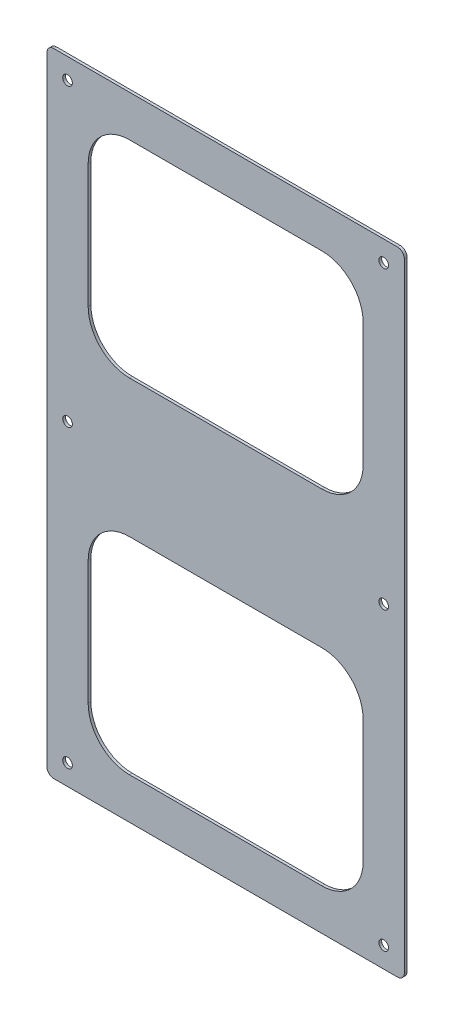
SolidWorks part; units mm, degrees
ref_plane "前视" through (0, 0, 0) normal (0, 0, 1) x (1, 0, 0)
ref_plane "上视" through (0, 0, 0) normal (0, 1, 0) x (1, 0, 0)
ref_plane "右视" through (0, 0, 0) normal (1, 0, 0) x (0, 0, -1)
sketch "草图1" plane through (0, 0, 0) normal (0, 0, 1) x (1, 0, 0)
  line L1 (0, 0) -> (260, 0)
  line L2 (0, 0) -> (0, -460)
  line L3 (0, -460) -> (260, -460)
  line L4 (260, 0) -> (260, -460)
  dimension "D1" = 260
  dimension "D2" = 460
extrude "凸台-拉伸1" add sketch "草图1" along normal blind 2
fillet "圆角1" radius 5 4 edges at (0, -460, 1) (260, -460, 1) (260, 0, 1) (0, 0, 1)
sketch "草图2" plane through (0, 0, 0) normal (0, 0, -1) x (-1, 0, 0)
  line L0 (-130, -460) -> (-130, 0) construction
  line L1 (-5, -460) -> (-255, -460) construction
  line L2 (-255, 0) -> (-5, 0) construction
  line L3 (0, -5) -> (0, -455) construction
  line L4 (-15, -445) -> (-245, -445) construction
  line L5 (-15, -445) -> (-15, -15) construction
  line L6 (-15, -15) -> (-245, -15) construction
  line L7 (-245, -445) -> (-245, -15) construction
  line L8 (-15, -445) -> (-245, -15) construction
  line L9 (-15, -15) -> (-245, -445) construction
  circle A0 centre (-245, -445) radius 3.5
  circle A1 centre (-15, -445) radius 3.5
  circle A2 centre (-245, -15) radius 3.5
  circle A3 centre (-15, -15) radius 3.5
  circle A5 centre (-245, -230) radius 3.5
  circle A7 centre (-15, -230) radius 3.5
  point P6 (-130, -230)
  dimension "D3" = 7
  dimension "D1" = 15
  dimension "D2" = 15
extrude "切除-拉伸1" cut sketch "草图2" against normal through all
sketch "草图3" plane through (0, 0, 0) normal (0, 0, -1) x (-1, 0, 0)
  line L3 (-60, -430) -> (-200, -430)
  line L4 (-60, -180) -> (-200, -180)
  line L5 (-30, -150) -> (-30, -60)
  line L6 (-60, -30) -> (-200, -30)
  line L7 (-230, -150) -> (-230, -60)
  line L8 (-30, -180) -> (-230, -30) construction
  line L9 (-30, -30) -> (-230, -180) construction
  line L10 (-30, -400) -> (-30, -310)
  line L11 (-60, -280) -> (-200, -280)
  line L12 (-230, -400) -> (-230, -310)
  line L13 (-30, -430) -> (-230, -280) construction
  line L14 (-30, -280) -> (-230, -430) construction
  line L15 (-260, -230) -> (-87.8187, -230) construction
  line L16 (-260, -455) -> (-260, -5) construction
  line L17 (-130, -460) -> (-130, 75.1002) construction
  line L18 (-5, -460) -> (-255, -460) construction
  arc A0 (-30, -60) -> (-60, -30) centre (-60, -60) ccw
  arc A1 (-200, -30) -> (-230, -60) centre (-200, -60) ccw
  arc A2 (-230, -150) -> (-200, -180) centre (-200, -150) ccw
  arc A3 (-60, -180) -> (-30, -150) centre (-60, -150) ccw
  arc A4 (-30, -310) -> (-60, -280) centre (-60, -310) ccw
  arc A5 (-200, -280) -> (-230, -310) centre (-200, -310) ccw
  arc A6 (-230, -400) -> (-200, -430) centre (-200, -400) ccw
  arc A7 (-60, -430) -> (-30, -400) centre (-60, -400) ccw
  point P2 (-130, -401.1105)
  point P6 (-130, -151.1105)
  dimension "D3" = 30
  dimension "D1" = 200
  dimension "D2" = 150
  dimension "D4" = 2
  dimension "D5" = 250
extrude "切除-拉伸2" cut sketch "草图3" against normal through all
